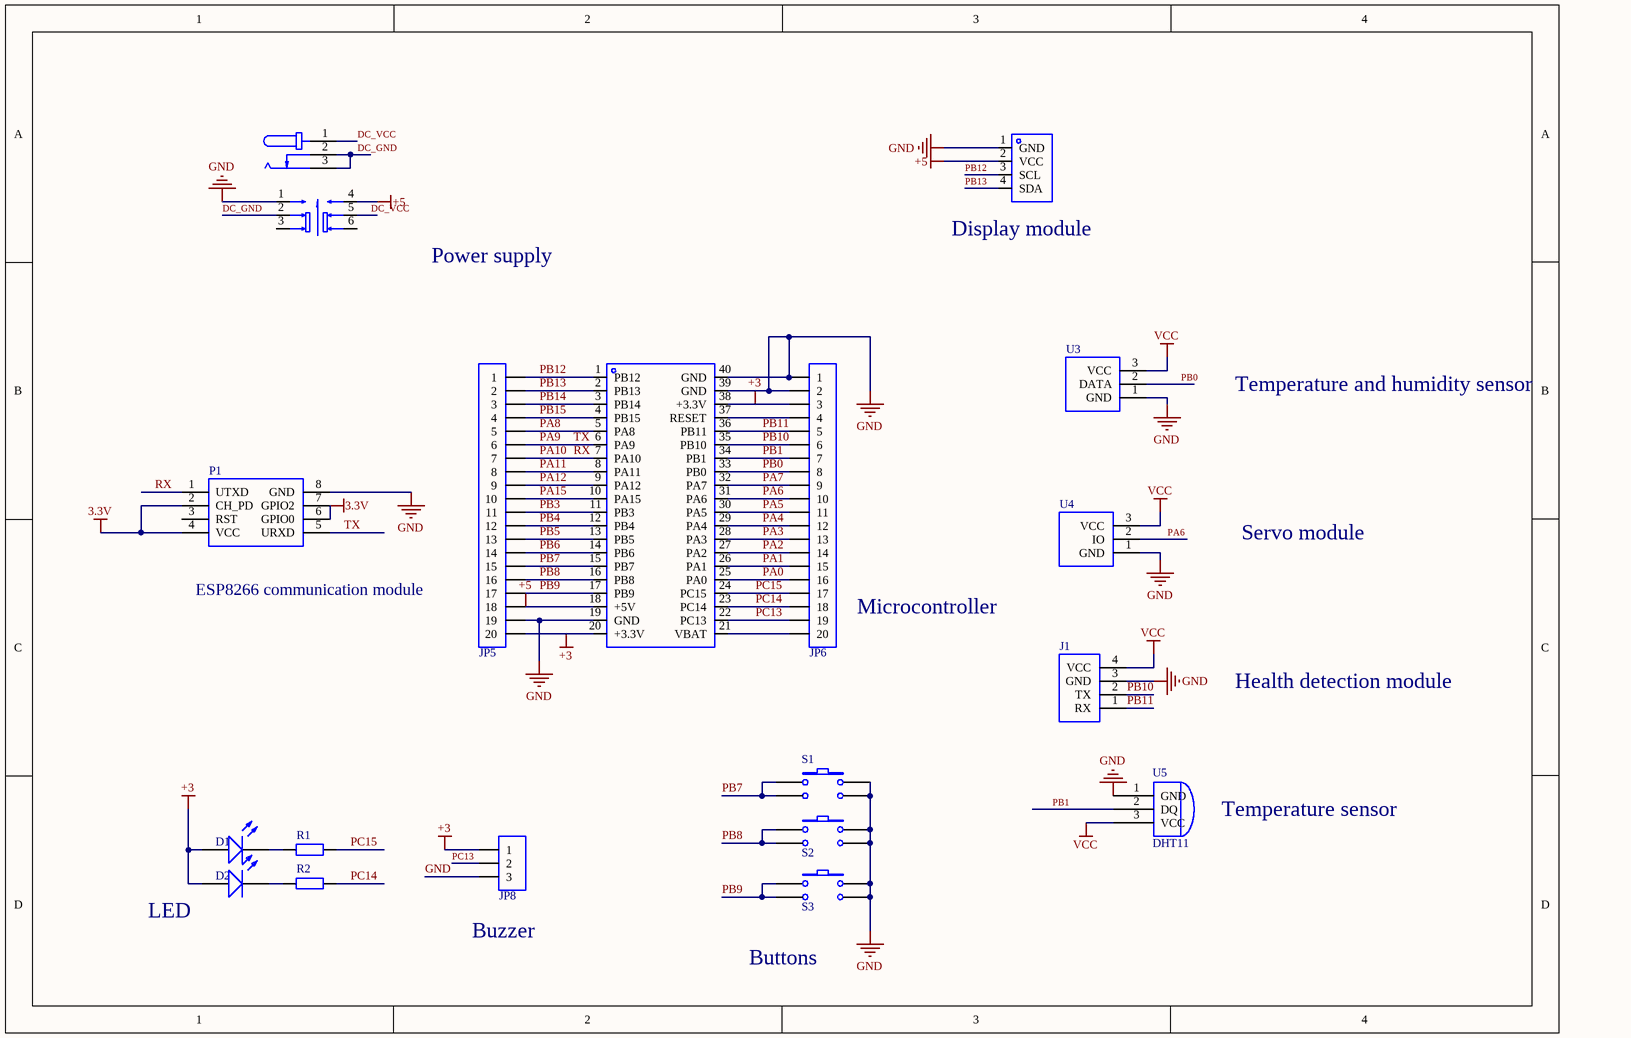
[diagram p0: MISC61251-3.schdoc]
# Altium project MISC61251-2.PrjPcb
1 sheet, 19 parts. Net scope: global (net labels, ports and power ports of the same name join across sheets).
Board file: MISC61251.pcbdoc

## Sheet MISC61251-3.schdoc
size 292 x 193 mm; SheetNumber: 1; SheetTotal: 1; Name: MISC61251

### Parts
D1  led  [LED-TH_5mm]  (value not drawn)
D2  led  [LED-TH_5mm]  (value not drawn)
DC1  DC002-1.3  [DC-IN-TH_DC002-1.3]  (value not drawn)
J1  (no value)  [HDR-TH_4P-P2.54-V-F]
JP5  HDR-1X20  [HDR-TH_20P-P2.54-V-F]  (value not drawn)
JP6  HDR-1X20  [HDR-TH_20P-P2.54-V-F-6]  (value not drawn)
JP8  HDR-1X3  [HDR-TH_3P-P2.54-V-F-4]  (value not drawn)
P1  (no value)  [ESP8266-1]
R1  Res2  [Res_1/8W]  (value not drawn)
R2  Res2  [Res_1/8W]  (value not drawn)
S1  key_4  [SW-TH_4P-L6.0-W6.0-P4.50-LS6.5]  (value not drawn)
S2  key_4  [SW-TH_4P-L6.0-W6.0-P4.50-LS6.5]  (value not drawn)
S3  key_4  [SW-TH_4P-L6.0-W6.0-P4.50-LS6.5]  (value not drawn)
SW1  Self-lock button  [SW-TH_6P-L7.0-W7.0-P2.00]  (value not drawn)
U1  OLED  [OLED-TH_L27.8-W27.2-P2.54_C9900033791]  (value not drawn)
U2  ST32F103C8T6  [CONN-TH_L53.3-W22.9_STM32F103C8T6-CARD]  (value not drawn)
U3  (no value)  [HDR-TH_3P-P2.54-V-F]
U4  (no value)  [HDR-TH_3P-P2.54-V-F]
U5  DHT11  [HDR-TH_3P-P2.54-V-F]

### Nets
3.3V: P1.2(CH_PD) P1.4(VCC) P1.6(GPIO0) P1.7(GPIO2)
+3: D1.1 D2.1 JP5.20 JP6.3 JP8.1 U2.20(+3.3V) U2.38(+3.3V)
+5: JP5.18 SW1.4 U1.2(VCC) U2.18(+5V)
GND: J1.3(GND) JP5.19 JP6.1 JP6.2 JP8.3 P1.8(GND) S1.2 S1.4 S2.2 S2.4 S3.2 S3.4 SW1.1 U1.1(GND) U2.19(GND) U2.39(GND) U2.40(GND) U3.1(GND) U4.1(GND) U5.1(GND)
VCC: J1.4(VCC) U3.3(VCC) U4.3(VCC) U5.3(VCC)
DC_GND: DC1.2 DC1.3 SW1.2
DC_VCC: DC1.1 SW1.5
PA0: JP6.16 U2.25(PA0)
PA1: JP6.15 U2.26(PA1)
PA2: JP6.14 U2.27(PA2)
PA3: JP6.13 U2.28(PA3)
PA4: JP6.12 U2.29(PA4)
PA5: JP6.11 U2.30(PA5)
PA6: JP6.10 U2.31(PA6) U4.2(IO)
PA7: JP6.9 U2.32(PA7)
PA8: JP5.5 U2.5(PA8)
PA9: JP5.6 P1.5(URXD) U2.6(PA9)  [also labelled TX]
PA10: JP5.7 P1.1(UTXD) U2.7(PA10)  [also labelled RX]
PA11: JP5.8 U2.8(PA11)
PA12: JP5.9 U2.9(PA12)
PA15: JP5.10 U2.10(PA15)
PB0: JP6.8 U2.33(PB0) U3.2(DATA)
PB1: JP6.7 U2.34(PB1) U5.2(DQ)
PB3: JP5.11 U2.11(PB3)
PB4: JP5.12 U2.12(PB4)
PB5: JP5.13 U2.13(PB5)
PB6: JP5.14 U2.14(PB6)
PB7: JP5.15 S1.1 S1.3 U2.15(PB7)
PB8: JP5.16 S2.1 S2.3 U2.16(PB8)
PB9: JP5.17 S3.1 S3.3 U2.17(PB9)
PB10: J1.2(TX) JP6.6 U2.35(PB10)
PB11: J1.1(RX) JP6.5 U2.36(PB11)
PB12: JP5.1 U1.3(SCL) U2.1(PB12)
PB13: JP5.2 U1.4(SDA) U2.2(PB13)
PB14: JP5.3 U2.3(PB14)
PB15: JP5.4 U2.4(PB15)
PC13: JP6.19 JP8.2 U2.22(PC13)
PC14: JP6.18 R2.2 U2.23(PC14)
PC15: JP6.17 R1.2 U2.24(PC15)
NetD1_2: D1.2 R1.1
NetD2_2: D2.2 R2.1
NetJP6_4: JP6.4 U2.37(RESET)
NetJP6_20: JP6.20 U2.21(VBAT)

Not connected (* = marked no-connect by the designer): P1 3(RST); SW1 3 6

### Notes on the sheet
- (near U1) Display module
- Power supply
- Temperature and humidity sensor
- Servo module
- ESP8266 communication module
- (near JP6) Microcontroller
- Health detection module
- Temperature sensor
- LED
- (near JP8) Buzzer
- (near S3) Buttons

### Library data of the parts
D1 = led: UniqueId: 07a0d5848cd81316; AddInBom: yes; Device: led; Origin Footprint: led; DesignItemID: led; LibraryName: Schlib1; SymbolName: led
D2 = led: UniqueId: fa5cd661465da5bc; AddInBom: yes; Device: led; Origin Footprint: led; DesignItemID: led; LibraryName: Schlib1; SymbolName: led
DC1 = DC002-1.3: Manufacturer: SHOU HAN(首韩); Add into BOM: yes; Connector Type: DC power jack; Inside Contact Diameter: 1.3mm; Outside Contact Diameter: 4.2mm; Current Rating (Max): 500mA; Voltage Rating (Max): 30V; UniqueId: 918354ff671956d3; ModelId: ccf1f99d79ab40ba9aeff26c21c7d5f1; Device: DC002-1.3; LCSC Part Name: DC电源插座 内径:1.3mm 外径:4.2mm; Supplier Part: C668593; Manufacturer Part: DC002-1.3; Supplier Footprint: 插件; JLCPCB Part Class: Extended Part; Datasheet: https://atta.szlcsc.com/upload/public/pdf/source/20200619/C668593_6B5785499F122503841AA69BD23A954B.pdf; Supplier: LCSC; Convert to PCB: yes; Mounting Style: Right angle; Operating Temperature Range: -; DesignItemID: DC002-1.3; LibraryName: Schlib1; SymbolName: DC002-1.3; FootprintName: DC-IN-TH_DC002-1.3; ModelName: DC-IN-TH_DC002-1.3
J1 = J1: Header, 4-Pin; Origin Footprint: HDR1X4; UniqueId: 9f49826860c2c79d; SymbolName: Header 4; AddInBom: yes; Device: J1; LatestRevisionDate: 17-Jul-2002; LatestRevisionNote: Re-released for DXP Platform.; DesignItemID: Header 4; LibraryName: Miscellaneous Connectors; Publisher: Altium Limited
JP5 = HDR-1X20: 20P connector; 学习资源: 最新版本发布; Origin Footprint: HDR2.54-LI-20P; UniqueId: 1fa703e6fb2f7410; SymbolName: Header 20; AddInBom: yes; Device: HDR-1X20; BOM名称: 20P connector; DesignItemID: Header 20; LibraryName: 5.4 - Connector - pitch 2.54 (100mil)
JP6 = HDR-1X20: 20P connector; 学习资源: 最新版本发布; Origin Footprint: HDR2.54-LI-20P; UniqueId: 93e224e006666394; SymbolName: Header 20; AddInBom: yes; Device: HDR-1X20; BOM名称: 20P connector; DesignItemID: Header 20; LibraryName: 5.4 - Connector - pitch 2.54 (100mil)
JP8 = HDR-1X3: 3P connector; 学习资源: 最新版本发布; Origin Footprint: HDR2.54-LI-3P; UniqueId: fe8a9be294322f66; SymbolName: Header 3; AddInBom: yes; Device: HDR-1X3; BOM名称: 3P connector; DesignItemID: Header 3; LibraryName: 5.4 - Connector - pitch 2.54 (100mil)
P1 = P1: Header, 5-Pin, Dual row; Value: ESP8266  WIFI模块+ 2*4P排座; Origin Footprint: ESP8266; UniqueId: f88e3064cb77b82c; SymbolName: wifi; AddInBom: yes; Device: P1; LatestRevisionDate: 17-Jul-2002; LatestRevisionNote: Re-released for DXP Platform.; DesignItemID: wifi; LibraryName: 20170808 graduation design module data; Publisher: Altium Limited
R1 = Res2: Resistor; Origin Footprint: AXIAL0.4-1/4W; UniqueId: 4e166b190d4de1c3; AddInBom: yes; Device: Res2; Published: 8-Jun-2000; LatestRevisionDate: 17-Jul-2002; LatestRevisionNote: Re-released for DXP Platform.; PackageReference: AXIAL-0.4; DesignItemID: Res2; LibraryName: Miscellaneous Devices; SymbolName: Res2; Publisher: Altium Limited
R2 = Res2: Resistor; Origin Footprint: AXIAL0.4-1/4W; UniqueId: 06442d24ab060343; AddInBom: yes; Device: Res2; Published: 8-Jun-2000; LatestRevisionDate: 17-Jul-2002; LatestRevisionNote: Re-released for DXP Platform.; PackageReference: AXIAL-0.4; DesignItemID: Res2; LibraryName: Miscellaneous Devices; SymbolName: Res2; Publisher: Altium Limited
S1 = key_4: UniqueId: da892dff24010eb4; AddInBom: yes; Device: key_4; Origin Footprint: key_4; DesignItemID: key_4; LibraryName: Schlib1; SymbolName: key_4
S2 = key_4: UniqueId: b3b756e6393b620b; AddInBom: yes; Device: key_4; Origin Footprint: key_4; DesignItemID: key_4; LibraryName: Schlib1; SymbolName: key_4
S3 = key_4: UniqueId: 7b79a888bb89fb64; AddInBom: yes; Device: key_4; Origin Footprint: key_4; DesignItemID: key_4; LibraryName: Schlib1; SymbolName: key_4
SW1 = 自锁按键: Manufacturer: XKB Connectivity(中国星坤); Manufacturer Part: XKB7070-Z; Add into BOM: yes; Actuator Style: Rectangular button; Contact Current: 100mA; Voltage Rating (AC): 250V; Voltage Rating (DC): 30V; Insulation Resistance: 100MΩ; Actuator/Cap Color: Blue; With Lamp: Without; Pin Style: PC pin; Operating Force: 160gf; Mechanical Life: 10万 times; UniqueId: 1070c7afd779bef2; ModelId: 65f5674ceb7247f197b01bc7adea0d8f; Device: Self-lock button; LCSC Part Name: 按键开关   7*7插件自锁 蓝白黑; Supplier Part: C318863; Supplier Footprint: 插件; JLCPCB Part Class: Extended Part; Datasheet: https://atta.szlcsc.com/upload/public/pdf/source/20211015/75A682A27A424BDE8D93C2CFA14C38FE.pdf; Supplier: LCSC; Convert to PCB: yes; Self Lock / No Lock: Self-lock; IP Rating: -; Mounting Style: Through hole; Operating Temperature: -15℃~+55℃; DesignItemID: XKB7070-Z; LibraryName: Schlib1; SymbolName: XKB7070-Z; FootprintName: SW-TH_6P-L7.0-W7.0-P2.00; ModelName: SW-TH_6P-L7.0-W7.0-P2.00
U1 = OLED: Manufacturer: HS(汉昇); Manufacturer Part: HS96L03W2C03; Add into BOM: yes; Main Control Chip: SSD1315; Interface Type: I2C; Pixel Resolution: 128x64; UniqueId: 48a4a086d8c42a18; SymbolName: OLED0.96; ModelId: bb65183306db4ca69fb52250be49b00e; Device: OLED; LCSC Part Name: 0.96寸OLED显示屏窄白光IIC; Supplier Part: C5248080; Supplier Footprint: -; JLCPCB Part Class: Extended Part; Datasheet: https://atta.szlcsc.com/upload/public/pdf/source/20230627/763D01F79A90007632F098068C7C8AD9.pdf; Supplier: LCSC; Convert to PCB: yes; Size: 0.96; Operating Temperature: -40℃~+70℃; DesignItemID: OLED0.96; LibraryName: Schlib1; FootprintName: OLED-TH_L27.8-W27.2-P2.54_C9900033791; ModelName: OLED-TH_L27.8-W27.2-P2.54_C9900033791
U2 = ST32F103C8T6: Manufacturer: 立创开发板; Manufacturer Part: LCKFB-DKX-STM32F103C8T6; Add into BOM: yes; UniqueId: d74c11912b695046; Device: ST32F103C8T6; LCSC Part Name: 立创·地阔星-STM32F103C8T6开发板; Supplier Part: C22396880; Supplier Footprint: -; Datasheet: https://atta.szlcsc.com/upload/public/pdf/source/20240801/7EEF69F7480DF7C6DA98696664D658D4.pdf; Supplier: LCSC; Convert to PCB: yes; Origin Footprint: ST32F103C8T6; DesignItemID: LCKFB-DKX-STM32F103C8T6; LibraryName: Schlib1; SymbolName: LCKFB-DKX-STM32F103C8T6
U3 = U3: Programmable digital thermometer; Part Number: E02P00451; Value: DS18B20; Power: 3~5.5V; MFG: MAXIM; Component: Standard; Origin Footprint: TO92; UniqueId: eac3f191c372887e; AddInBom: yes; Device: U3; Part Type: Other; MPN: DS18B20; Price: 4.1; Availability: A; Temperature: -45°C ~ 125°C; ComponentLink1Description: Datasheet; DesignItemID: E02P00451; LibraryName: Library; SymbolName: E02P00451
U4 = U4: Programmable digital thermometer; Part Number: E02P00451; Value: DS18B20; Power: 3~5.5V; MFG: MAXIM; Component: Standard; Origin Footprint: TO92; UniqueId: e5d1bee62801ccc5; AddInBom: yes; Device: U4; Part Type: Other; MPN: DS18B20; Price: 4.1; Availability: A; Temperature: -45°C ~ 125°C; ComponentLink1Description: Datasheet; DesignItemID: E02P00451; LibraryName: Library; SymbolName: E02P00451
U5 = DHT11: Origin Footprint: SIP3; UniqueId: 65fd737caad1a168; SymbolName: DS18B20; AddInBom: yes; Device: DHT11; DesignItemID: DS18B20; LibraryName: *